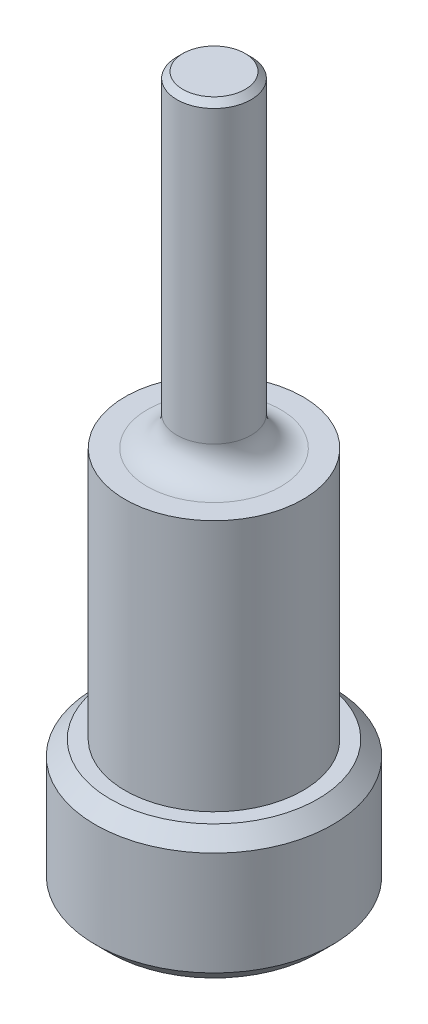
from build123d import *

# Parameters (mm, degrees)
CHAMFER_1_SIZE = 0.5
FILLET_1_R     = 1
CHAMFER_2_SIZE = 0.2


with BuildPart() as part:
    # 草图1 → 旋转1 (revolve)
    with BuildSketch(Plane.XY, mode=Mode.PRIVATE) as revolve_1_sk:
        Polygon((1.25, 24), (1.25, 13), (3, 13), (3, 4.5), (4, 4.5), (4, 0), (0, 0), (0, 24), align=None)
    revolve(revolve_1_sk.sketch.rotate(Axis((0, -0.524377328, 0), (0, 1, 0)), 90), axis=Axis((0, -0.524377328, 0), (0, 1, 0)))

    # 倒角1
    chamfer_1_edges = [part.edges().sort_by_distance(p)[0] for p in [
        (0, 0, 4),
        (0, 4.5, 4),
    ]]
    chamfer(chamfer_1_edges, length=CHAMFER_1_SIZE)

    # 圆角1
    fillet_1_edges = [part.edges().sort_by_distance(p)[0] for p in [
        (0, 13, 1.25),
    ]]
    fillet(fillet_1_edges, radius=FILLET_1_R)

    # 倒角2
    chamfer_2_edges = [part.edges().sort_by_distance(p)[0] for p in [
        (0, 24, 1.25),
    ]]
    chamfer(chamfer_2_edges, length=CHAMFER_2_SIZE)


solid = part.part
